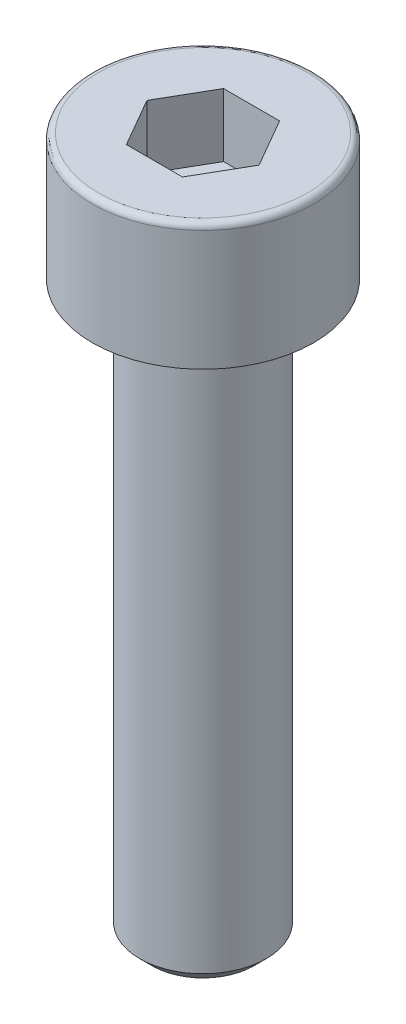
from build123d import *

# Parameters (mm, degrees)
SKETCH_1_R          = 3.5
EXTRUDE_1_DEPTH     = 4
CUT_EXTRUDE_1_DEPTH = 2
FILLET_1_R          = 0.2
SKETCH_5_R          = 2
EXTRUDE_2_DEPTH     = 18
CHAMFER_2_SIZE      = 0.39


with BuildPart() as part:
    # 草图1 → 凸台-拉伸1 (new body)
    with BuildSketch(Plane(origin=(0, 0, 0), x_dir=(1, 0, 0), z_dir=(0, 1, 0))):
        with Locations(Location((0, 0, 0), (0, 0, 270))):
            Circle(SKETCH_1_R)
    extrude(amount=EXTRUDE_1_DEPTH)

    # 草图2 → 切除-拉伸1 (cut)
    with BuildSketch(Plane(origin=(0, 4, 0), x_dir=(1, 0, 0), z_dir=(0, 1, 0))):
        Polygon((1.772465326, 0), (0.886232663, 1.535), (-0.886232663, 1.535), (-1.772465326, 0), (-0.886232663, -1.535), (0.886232663, -1.535), align=None)
    extrude(amount=-CUT_EXTRUDE_1_DEPTH, mode=Mode.SUBTRACT)

    # 圆角1
    fillet_1_edges = [part.edges().sort_by_distance(p)[0] for p in [
        (0, 4, -3.5),
    ]]
    fillet(fillet_1_edges, radius=FILLET_1_R)

    # 草图5 → 凸台-拉伸2 (add)
    with BuildSketch(Plane.XZ):
        with Locations(Location((0, 0, 0), (0, 0, 90))):
            Circle(SKETCH_5_R)
    extrude(amount=EXTRUDE_2_DEPTH)

    # 倒角2
    chamfer_2_edges = [part.edges().sort_by_distance(p)[0] for p in [
        (0, -18, -2),
    ]]
    chamfer(chamfer_2_edges, length=CHAMFER_2_SIZE)


solid = part.part
